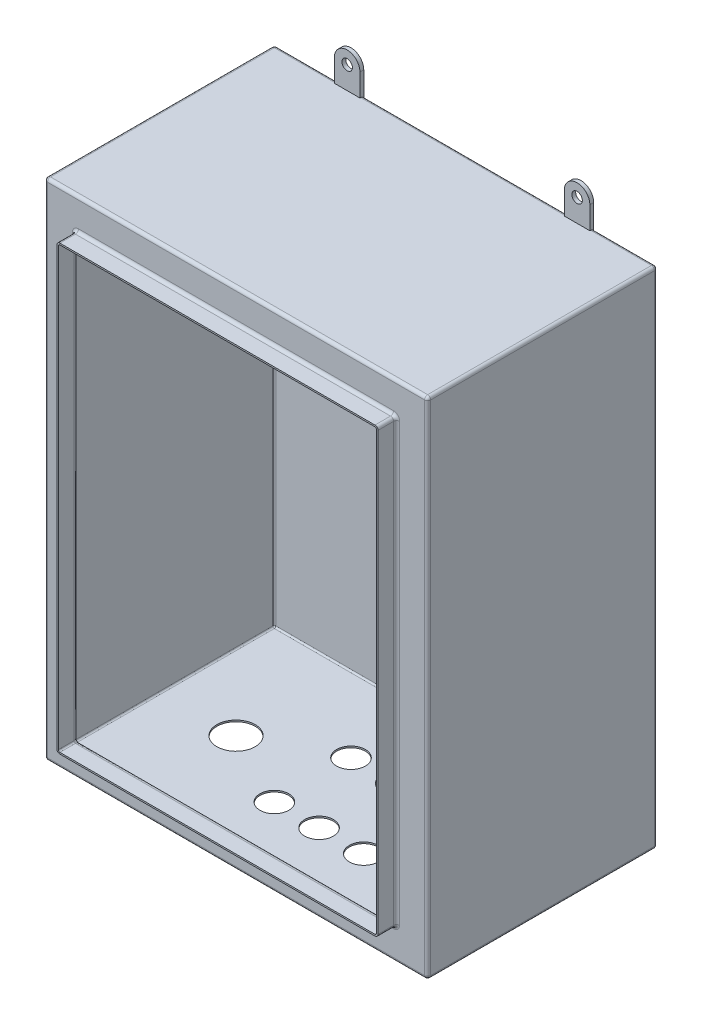
from build123d import *

# Parameters (mm, degrees)
SKETCH1_W           = 300
SKETCH1_H           = 180
BOSS_EXTRUDE1_DEPTH = 395
FILLET1_R           = 2.4
SKETCH2_W           = 251.48
SKETCH2_H           = 346.48
BOSS_EXTRUDE2_DEPTH = 14.57
FILLET2_R           = 2.4
SHELL1_T            = -1.2
SKETCH3_R           = 15
SKETCH3_R_2         = 11.25
CUT_EXTRUDE1_DEPTH  = 435.181212053
SKETCH4_R           = 4.1
BOSS_EXTRUDE3_DEPTH = 3


with BuildPart() as part:
    # Sketch1 → Boss-Extrude1 (new body)
    with BuildSketch(Plane(origin=(0, 0, 0), x_dir=(1, 0, 0), z_dir=(0, 1, 0))):
        Rectangle(SKETCH1_W, SKETCH1_H)
    extrude(amount=BOSS_EXTRUDE1_DEPTH)

    # Fillet1
    fillet1_edges = [part.edges().sort_by_distance(p)[0] for p in [
        (-150, 395, 0),
        (0, 395, 90),
        (150, 395, 0),
        (0, 0, 90),
        (-150, 0, 0),
        (0, 0, -90),
        (150, 0, 0),
        (0, 395, -90),
        (150, 197.5, 90),
        (-150, 197.5, 90),
        (-150, 197.5, -90),
        (150, 197.5, -90),
    ]]
    fillet(fillet1_edges, radius=FILLET1_R)

    # Sketch2 → Boss-Extrude2 (add)
    with BuildSketch(Plane.XY.offset(90)):
        with Locations((0, 197.5)):
            Rectangle(SKETCH2_W, SKETCH2_H)
    extrude(amount=BOSS_EXTRUDE2_DEPTH)

    # Fillet2
    fillet2_edges = [part.edges().sort_by_distance(p)[0] for p in [
        (-125.74, 197.5, 90),
        (-125.74, 370.74, 97.285),
        (0, 24.26, 90),
        (-125.74, 24.26, 97.285),
        (125.74, 197.5, 90),
        (125.74, 24.26, 97.285),
        (0, 370.74, 90),
        (125.74, 370.74, 97.285),
    ]]
    fillet(fillet2_edges, radius=FILLET2_R)

    # Shell1
    shell1_openings = [part.faces().sort_by_distance(p)[0] for p in [
        (0, 197.5, 104.57),
    ]]
    offset(amount=SHELL1_T, openings=shell1_openings, kind=Kind.INTERSECTION)

    # Sketch3 → Cut-Extrude1 (cut, through all)
    with BuildSketch(Plane(origin=(0, 1.2, 0), x_dir=(1, 0, 0), z_dir=(0, 1, 0))):
        with Locations(Location((-90, 0, 0), (0, 0, 270))):
            Circle(SKETCH3_R)
        with Locations(Location((-30, -30, 0), (0, 0, 270))):
            Circle(SKETCH3_R_2)
        with Locations(Location((-30, 30, 0), (0, 0, 270))):
            Circle(SKETCH3_R_2)
        with Locations(Location((5, -30, 0), (0, 0, 270))):
            Circle(SKETCH3_R_2)
        with Locations(Location((5, 30, 0), (0, 0, 270))):
            Circle(SKETCH3_R_2)
        with Locations(Location((40, -30, 0), (0, 0, 270))):
            Circle(SKETCH3_R_2)
        with Locations(Location((40, 30, 0), (0, 0, 270))):
            Circle(SKETCH3_R_2)
        with Locations(Location((75, -30, 0), (0, 0, 270))):
            Circle(SKETCH3_R_2)
        with Locations(Location((75, 30, 0), (0, 0, 270))):
            Circle(SKETCH3_R_2)
    extrude(amount=-CUT_EXTRUDE1_DEPTH, mode=Mode.SUBTRACT)

    # Sketch4 → Boss-Extrude3 (add)
    # profile 1 of 4: a face of its own
    with BuildSketch(Plane(origin=(0, 0, -90), x_dir=(-1, 0, 0), z_dir=(0, 0, -1))):
        with BuildLine():
            Line((-100, 412.6), (-100, 393.8))
            Line((-100, 393.8), (-80, 393.8))
            Line((-80, 393.8), (-80, 412.6))
            ThreePointArc((-80, 412.6), (-90, 422.6), (-100, 412.6))
        make_face()
        with Locations((-90, 412.6)):
            Circle(SKETCH4_R, mode=Mode.SUBTRACT)
    # profile 2 of 4: a face of its own
    with BuildSketch(Plane(origin=(0, 0, -90), x_dir=(-1, 0, 0), z_dir=(0, 0, -1))):
        with BuildLine():
            Line((80, 412.6), (80, 393.8))
            Line((80, 393.8), (100, 393.8))
            Line((100, 393.8), (100, 412.6))
            ThreePointArc((100, 412.6), (90, 422.6), (80, 412.6))
        make_face()
        with Locations((90, 412.6)):
            Circle(SKETCH4_R, mode=Mode.SUBTRACT)
    # profile 3 of 4: a face of its own
    with BuildSketch(Plane(origin=(0, 0, -90), x_dir=(-1, 0, 0), z_dir=(0, 0, -1))):
        with BuildLine():
            Line((-100, 1.2), (-100, -12.530239685))
            ThreePointArc((-100, -12.530239685), (-90, -22.530239685), (-80, -12.530239685))
            Line((-80, -12.530239685), (-80, 1.2))
            Line((-80, 1.2), (-100, 1.2))
        make_face()
        with Locations((-90, -12.530239685)):
            Circle(SKETCH4_R, mode=Mode.SUBTRACT)
    # profile 4 of 4: a face of its own
    with BuildSketch(Plane(origin=(0, 0, -90), x_dir=(-1, 0, 0), z_dir=(0, 0, -1))):
        with BuildLine():
            Line((80, 1.2), (80, -12.530239685))
            ThreePointArc((80, -12.530239685), (90, -22.530239685), (100, -12.530239685))
            Line((100, -12.530239685), (100, 1.2))
            Line((100, 1.2), (80, 1.2))
        make_face()
        with Locations((90, -12.530239685)):
            Circle(SKETCH4_R, mode=Mode.SUBTRACT)
    extrude(amount=-BOSS_EXTRUDE3_DEPTH)


solid = part.part
